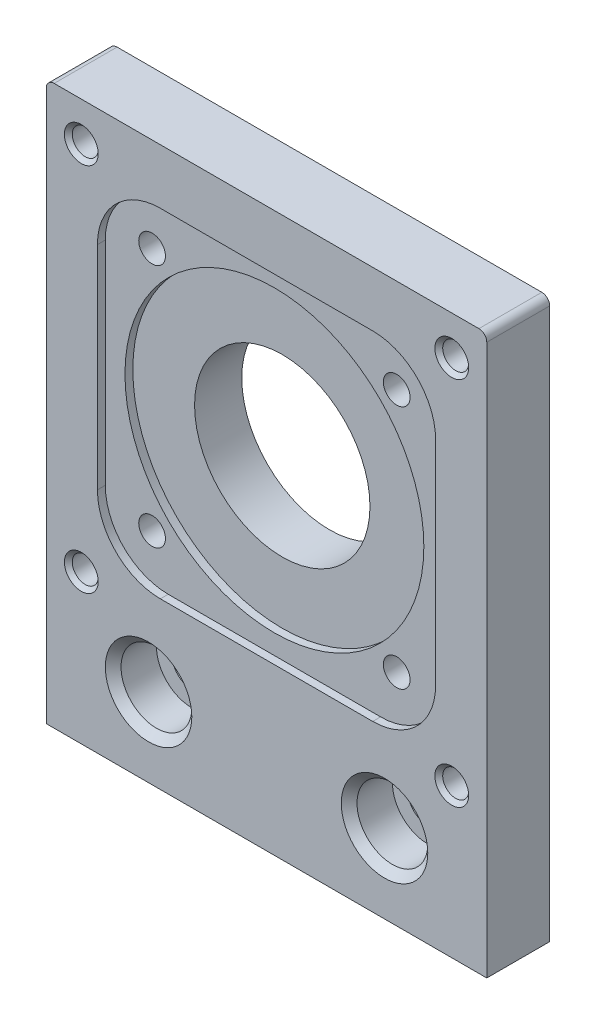
from build123d import *

# Parameters (mm, degrees)
SKETCH1_R           = 11.15
SKETCH1_R_2         = 1.7
SKETCH1_R_3         = 1
SKETCH1_R_4         = 2.5
BOSS_EXTRUDE1_DEPTH = 8
SKETCH2_R           = 4.5
CUT_EXTRUDE1_DEPTH  = 5.5
SKETCH3_R           = 3
CUT_EXTRUDE2_DEPTH  = 4
CHAMFER1_SIZE       = 1
CHAMFER2_SIZE       = 0.5
CHAMFER3_SIZE       = 0.5
SKETCH4_R           = 19
CUT_EXTRUDE3_DEPTH  = 2
CUT_EXTRUDE4_DEPTH  = 1
CHAMFER4_SIZE       = 1
M4_TAPPED_HOLE1_D   = 3.3
CHAMFER5_SIZE       = 0.5


with BuildPart() as part:
    # Sketch1 → Boss-Extrude1 (new body)
    with BuildSketch(Plane.XY):
        with BuildLine():
            Line((-27, 35.5), (27, 35.5))
            ThreePointArc((27, 35.5), (27.707106781, 35.207106781), (28, 34.5))
            Line((28, 34.5), (28, -35.5))
            Line((28, -35.5), (-28, -35.5))
            Line((-28, -35.5), (-28, 34.5))
            ThreePointArc((-28, 34.5), (-27.707106781, 35.207106781), (-27, 35.5))
        make_face()
        with Locations((0, 7)):
            Circle(SKETCH1_R, mode=Mode.SUBTRACT)
        with Locations((-15.55, 22.55)):
            Circle(SKETCH1_R_2, mode=Mode.SUBTRACT)
        with Locations((-23.55, 30.55)):
            Circle(SKETCH1_R_3, mode=Mode.SUBTRACT)
        with Locations(Location((23.55, 30.55, 0), (0, 0, 180))):
            Circle(SKETCH1_R_3, mode=Mode.SUBTRACT)
        with Locations(Location((15.55, 22.55, 0), (0, 0, 180))):
            Circle(SKETCH1_R_2, mode=Mode.SUBTRACT)
        with Locations(Location((-23.55, -16.55, 0), (0, 0, 180))):
            Circle(SKETCH1_R_3, mode=Mode.SUBTRACT)
        with Locations(Location((-15.55, -8.55, 0), (0, 0, 180))):
            Circle(SKETCH1_R_2, mode=Mode.SUBTRACT)
        with Locations((15.55, -8.55)):
            Circle(SKETCH1_R_2, mode=Mode.SUBTRACT)
        with Locations((23.55, -16.55)):
            Circle(SKETCH1_R_3, mode=Mode.SUBTRACT)
        with Locations((-15, -25.5)):
            Circle(SKETCH1_R_4, mode=Mode.SUBTRACT)
        with Locations((15, -25.5)):
            Circle(SKETCH1_R_4, mode=Mode.SUBTRACT)
    extrude(amount=BOSS_EXTRUDE1_DEPTH)

    # Sketch2 → Cut-Extrude1 (cut)
    with BuildSketch(Plane.XY.offset(8)):
        with Locations((-15, -25.5)):
            Circle(SKETCH2_R)
        with Locations((15, -25.5)):
            Circle(SKETCH2_R)
    extrude(amount=-CUT_EXTRUDE1_DEPTH, mode=Mode.SUBTRACT)

    # Sketch3 → Cut-Extrude2 (cut)
    with BuildSketch(Plane(origin=(0, 0, 0), x_dir=(-1, 0, 0), z_dir=(0, 0, -1))):
        with Locations((-15.55, 22.55)):
            Circle(SKETCH3_R)
        with Locations((15.55, 22.55)):
            Circle(SKETCH3_R)
        with Locations((-15.55, -8.55)):
            Circle(SKETCH3_R)
        with Locations((15.55, -8.55)):
            Circle(SKETCH3_R)
    extrude(amount=-CUT_EXTRUDE2_DEPTH, mode=Mode.SUBTRACT)

    # Chamfer1
    chamfer1_edges = [part.edges().sort_by_distance(p)[0] for p in [
        (18.55, 22.55, 0),
        (-12.55, 22.55, 0),
        (18.55, -8.55, 0),
        (-12.55, -8.55, 0),
    ]]
    chamfer(chamfer1_edges, length=CHAMFER1_SIZE)

    # Chamfer2
    chamfer2_edges = [part.edges().sort_by_distance(p)[0] for p in [
        (-24.55, 30.55, 0),
        (24.55, 30.55, 0),
        (-22.55, -16.55, 0),
        (22.55, -16.55, 0),
    ]]
    chamfer(chamfer2_edges, length=CHAMFER2_SIZE)

    # Chamfer3
    chamfer3_edges = [part.edges().sort_by_distance(p)[0] for p in [
        (-24.55, 30.55, 8),
        (24.55, 30.55, 8),
        (-22.55, -16.55, 8),
        (22.55, -16.55, 8),
    ]]
    chamfer(chamfer3_edges, length=CHAMFER3_SIZE)

    # Sketch4 → Cut-Extrude3 (cut)
    with BuildSketch(Plane.XY.offset(8)):
        with Locations((0, 7)):
            Circle(SKETCH4_R)
    extrude(amount=-CUT_EXTRUDE3_DEPTH, mode=Mode.SUBTRACT)

    # Sketch5 → Cut-Extrude4 (cut)
    with BuildSketch(Plane.XY.offset(8)):
        with BuildLine():
            Line((-13.5, 28.5), (13.5, 28.5))
            ThreePointArc((13.5, 28.5), (19.156854249, 26.156854249), (21.5, 20.5))
            Line((21.5, 20.5), (21.5, -6.5))
            ThreePointArc((21.5, -6.5), (19.156854249, -12.156854249), (13.5, -14.5))
            Line((13.5, -14.5), (-13.5, -14.5))
            ThreePointArc((-13.5, -14.5), (-19.156854249, -12.156854249), (-21.5, -6.5))
            Line((-21.5, -6.5), (-21.5, 20.5))
            ThreePointArc((-21.5, 20.5), (-19.156854249, 26.156854249), (-13.5, 28.5))
        make_face()
    extrude(amount=-CUT_EXTRUDE4_DEPTH, mode=Mode.SUBTRACT)

    # Chamfer4
    chamfer4_edges = [part.edges().sort_by_distance(p)[0] for p in [
        (-19.5, -25.5, 8),
        (10.5, -25.5, 8),
    ]]
    chamfer(chamfer4_edges, length=CHAMFER4_SIZE)

    # M4 Tapped Hole1 (through all)
    with Locations(Plane.XY.offset(8)):
        with Locations((-23.55, 30.55), (23.55, 30.55), (23.55, -16.55), (-23.55, -16.55)):
            Hole(M4_TAPPED_HOLE1_D / 2)

    # Chamfer5
    chamfer5_edges = [part.edges().sort_by_distance(p)[0] for p in [
        (-21.9, -16.55, 8),
        (-21.9, -16.55, 0),
        (25.2, -16.55, 8),
        (25.2, -16.55, 0),
        (25.2, 30.55, 8),
        (25.2, 30.55, 0),
        (-21.9, 30.55, 8),
        (-21.9, 30.55, 0),
    ]]
    chamfer(chamfer5_edges, length=CHAMFER5_SIZE)


solid = part.part
